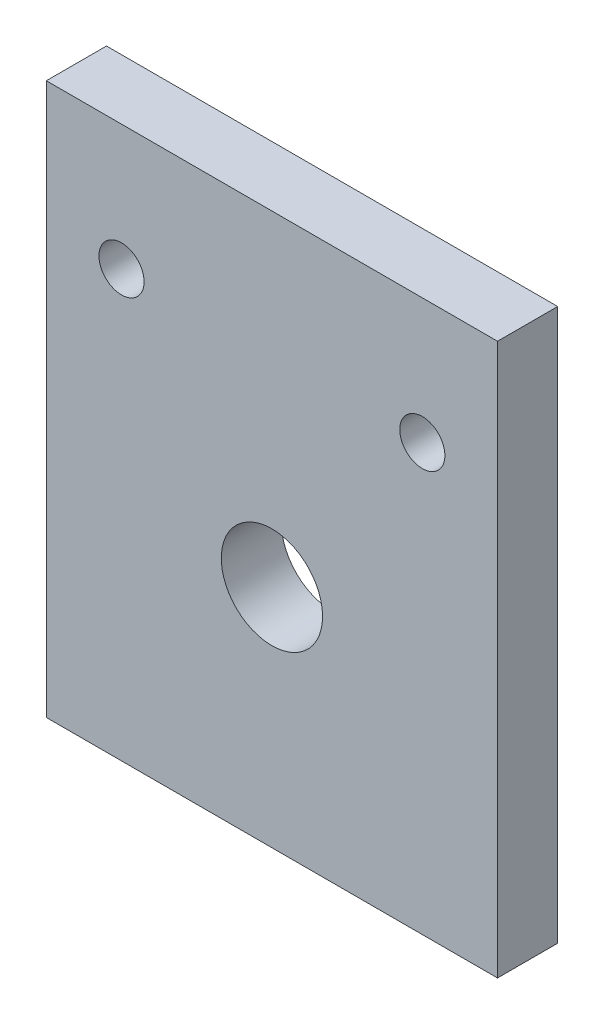
from build123d import *

# Parameters (mm, degrees)
SKETCH_1_W          = 90
SKETCH_1_H          = 110
EXTRUDE_1_DEPTH     = 6
SKETCH_2_R          = 4.5
SKETCH_2_R_2        = 10.1
CUT_EXTRUDE_1_DEPTH = 16


with BuildPart() as part:
    # 草图1 → 凸台-拉伸1 (new, symmetric)
    with BuildSketch(Plane.XY):
        Rectangle(SKETCH_1_W, SKETCH_1_H)
    extrude(amount=EXTRUDE_1_DEPTH, both=True)

    # 草图2 → 切除-拉伸1 (cut, symmetric)
    with BuildSketch(Plane.XY):
        with Locations((-30, 30)):
            Circle(SKETCH_2_R)
        with Locations((30, 30)):
            Circle(SKETCH_2_R)
        with Locations((0, -10)):
            Circle(SKETCH_2_R_2)
    extrude(amount=CUT_EXTRUDE_1_DEPTH, both=True, mode=Mode.SUBTRACT)


solid = part.part
